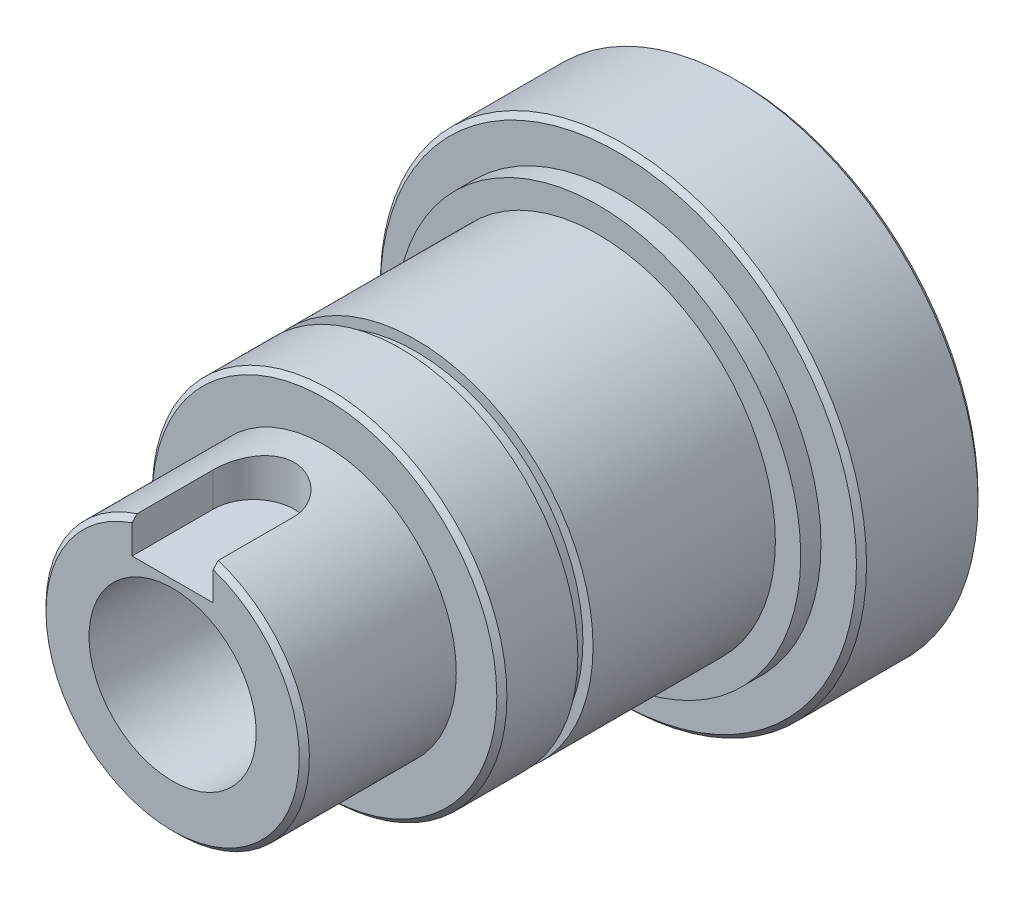
SolidWorks part; units mm, degrees
material "S45C"
ref_plane "Front Plane" through (0, 0, 0) normal (0, 0, 1) x (1, 0, 0)
ref_plane "Top Plane" through (0, 0, 0) normal (0, 1, 0) x (1, 0, 0)
ref_plane "Right Plane" through (0, 0, 0) normal (1, 0, 0) x (0, 0, -1)
sketch "Sketch1" plane through (0, 0, 0) normal (0, 0, 1) x (1, 0, 0)
  circle A0 centre (0, 0) radius 24
  dimension "D1" = 48
extrude "Boss-Extrude1" add sketch "Sketch1" along normal blind 12
sketch "Sketch2" plane through (0, 0, 12) normal (0, 0, 1) x (1, 0, 0)
  circle A0 centre (0, 0) radius 20
  dimension "D1" = 40
extrude "Boss-Extrude2" add sketch "Sketch2" along normal blind 2
sketch "Sketch3" plane through (0, 0, 14) normal (0, 0, 1) x (1, 0, 0)
  circle A0 centre (0, 0) radius 17.5
  dimension "D1" = 35
extrude "Boss-Extrude3" add sketch "Sketch3" along normal blind 27
sketch "Sketch4" plane through (0, 0, 41) normal (0, 0, 1) x (1, 0, 0)
  circle A0 centre (0, 0) radius 13
  dimension "D1" = 26
extrude "Boss-Extrude4" add sketch "Sketch4" along normal blind 15
sketch "Sketch5" plane through (0, 0, 0) normal (0, 0, -1) x (-1, 0, 0)
  circle A0 centre (0, 0) radius 14
  dimension "D1" = 28
extrude "Cut-Extrude1" cut sketch "Sketch5" against normal blind 37.1
sketch "Sketch6" plane through (0, 0, 56) normal (0, 0, 1) x (1, 0, 0)
  circle A0 centre (0, 0) radius 8.25
  dimension "D1" = 16.5
extrude "Cut-Extrude2" cut sketch "Sketch6" against normal through all
ref_plane "Plane1" through (0, 13, 0) normal (0, 1, 0) x (1, 0, 0)
sketch "Sketch7" plane through (0, 13, 0) normal (0, 1, 0) x (1, 0, 0)
  line L0 (0, -48) -> (0, -64) construction
  line L1 (4, -48) -> (4, -64)
  line L2 (-4, -48) -> (-4, -64)
  line L4 (-13, -56) -> (13, -56) construction
  arc A0 (4, -48) -> (-4, -48) centre (0, -48) ccw
  arc A1 (-4, -64) -> (4, -64) centre (0, -64) ccw
  point P2 (0, -56)
  dimension "D1" = 4
  dimension "D2" = 16
extrude "Cut-Extrude3" cut sketch "Sketch7" against normal blind 4
sketch "Sketch8" plane through (0, 0, 41) normal (0, 0, 1) x (1, 0, 0)
  circle A0 centre (0, 0) radius 16.5
  circle A1 centre (0, 0) radius 29.2164
  dimension "D1" = 33
extrude "Cut-Extrude4" cut sketch "Sketch8" against normal blind 1.5 from offset 7.5 offset against normal yes
hole_wizard "M5 Tapped Hole1" positions "Sketch9" profile "Sketch10" tap size "M5" standard "ISO"
sketch "Sketch9" plane through (0, 0, 0) normal (0, 0, -1) x (-1, 0, 0)
  line L0 (0, 0) -> (0, 27.5154) construction
  line L2 (0, 0) -> (-20.4659, 20.4659) construction
  line L3 (0, 0) -> (5.2203, 0) construction
  circle A0 centre (0, 0) radius 19 construction
  point P0 (0, 19)
  point P18 (-13.435, 13.435)
  point P23 (13.435, 13.435)
  point P31 (-13.435, -13.435)
  point P32 (0, -19)
  point P33 (13.435, -13.435)
  dimension "D1" = 38
  dimension "D2" = 45
sketch "Sketch10" plane through (0, 19, 0) normal (1, 0, 0) x (0, 1, 0)
  line L0 (0, 0) -> (0, 11.2618)
  line L1 (0, 11.2618) -> (2.1, 10)
  line L2 (2.1, 10) -> (2.1, 0)
  line L5 (2.1, 0) -> (0, 0)
  line L10 (0, 11.2618) -> (-2.1, 10) construction
  line L11 (0, -6.35) -> (0, 107.95) construction
  dimension "螺纹孔钻头直径" = 4.2
  dimension "螺纹孔钻头深度" = 10
  dimension "导头角度" = 118
cosmetic thread "Cosmetic thread1" parameters "D1"=10, "D2"=5
cosmetic thread "Cosmetic thread2" parameters "D1"=10, "D2"=5
cosmetic thread "Cosmetic thread3" parameters "D1"=10, "D2"=5
cosmetic thread "Cosmetic thread4" parameters "D1"=10, "D2"=5
cosmetic thread "Cosmetic thread5" parameters "D1"=10, "D2"=5
cosmetic thread "Cosmetic thread6" parameters "D1"=10, "D2"=5
chamfer "Chamfer1" distance 0.5 angle 45 4 edges at (17.5, 0, 41) (24, 0, 12) (24, 0, 0) (0, -13, 56)
